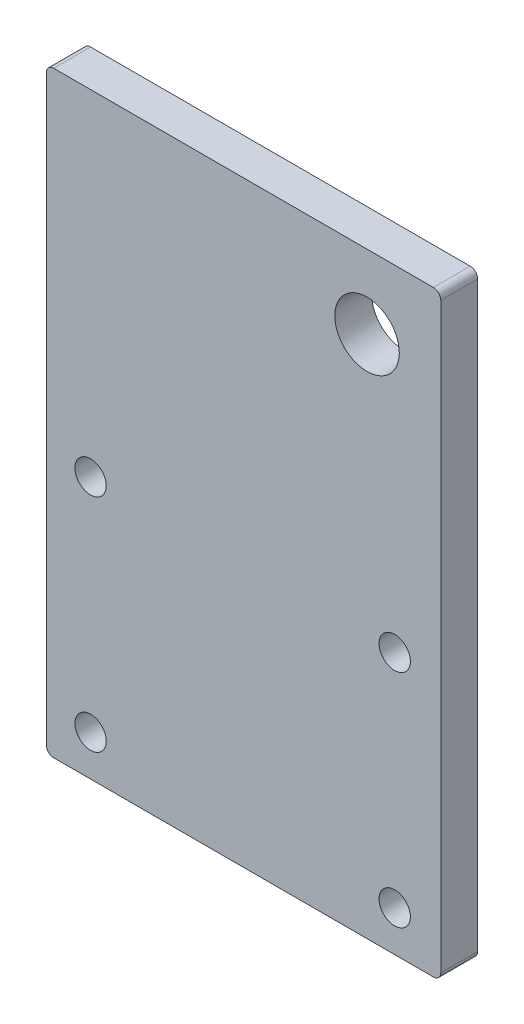
from build123d import *

# Parameters (mm, degrees)
SKETCH_1_W                  = 107
SKETCH_1_H                  = 162
EXTRUDE_1_DEPTH             = 5
HOLE_WIZARD_M20_1_D         = 17.5
FILLET_1_R                  = 2
HOLE_WIZARD_M10_1_D         = 8.5
PATTERN_LINEAR_1_COUNT      = 2
PATTERN_LINEAR_1_PITCH      = 82.5
PATTERN_LINEAR_1_COUNT_DIR2 = 2
PATTERN_LINEAR_1_PITCH_DIR2 = 60


with BuildPart() as part:
    # 草图1 → 凸台-拉伸1 (new, symmetric)
    with BuildSketch(Plane.XY):
        Rectangle(SKETCH_1_W, SKETCH_1_H)
    extrude(amount=EXTRUDE_1_DEPTH, both=True)

    # M20 螺纹孔1 (through all)
    with Locations(Plane.XY.offset(5)):
        with Locations((33.5, 61)):
            Hole(HOLE_WIZARD_M20_1_D / 2)

    # 圆角1
    fillet_1_edges = [part.edges().sort_by_distance(p)[0] for p in [
        (53.5, -81, 0),
        (-53.5, -81, 0),
        (-53.5, 81, 0),
        (53.5, 81, 0),
    ]]
    fillet(fillet_1_edges, radius=FILLET_1_R)

    # M10 螺纹孔1 (through all)
    with Locations(Plane.XY.offset(5)):
        with Locations((-41.5, -70)):
            hole_wizard_m10_1 = Hole(HOLE_WIZARD_M10_1_D / 2)

    # 阵列(线性)1: Hole Wizard M10 _1 2 × 2
    with Locations(*[(i * PATTERN_LINEAR_1_PITCH, j * PATTERN_LINEAR_1_PITCH_DIR2, 0) for i in range(PATTERN_LINEAR_1_COUNT) for j in range(PATTERN_LINEAR_1_COUNT_DIR2) if (i, j) != (0, 0)]):
        add(hole_wizard_m10_1, mode=Mode.SUBTRACT)


solid = part.part
